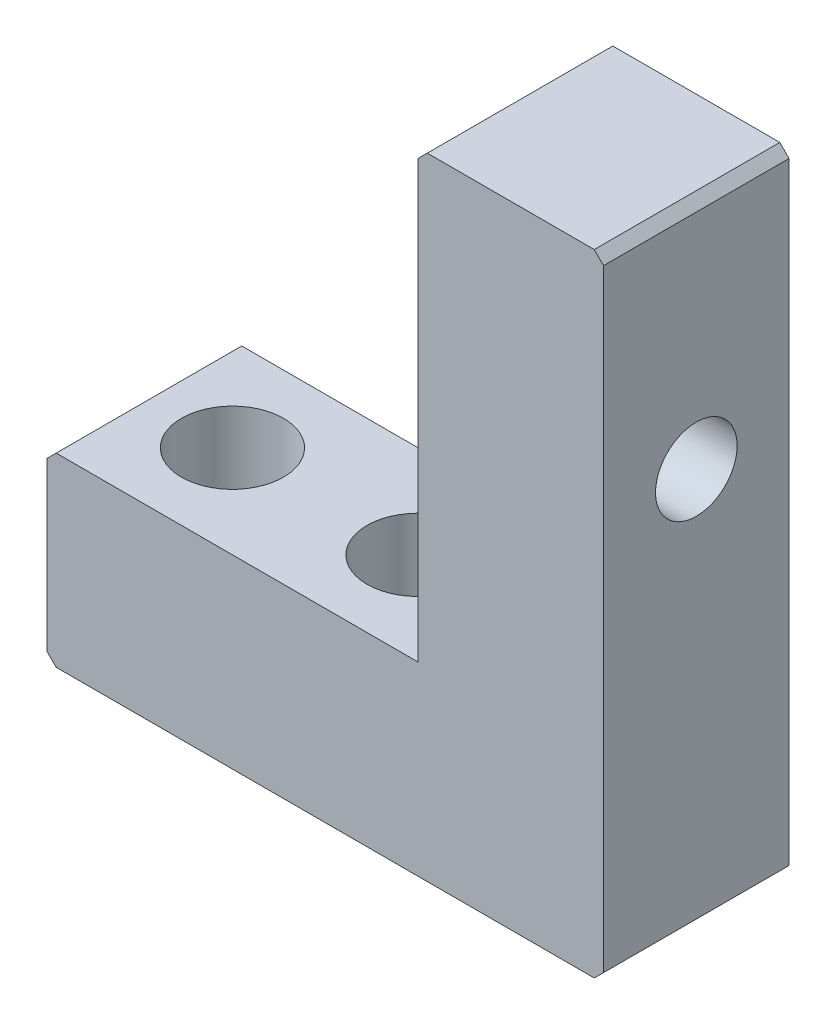
SolidWorks part; units mm, degrees
ref_plane "Front Plane" through (0, 0, 0) normal (0, 0, 1) x (1, 0, 0)
ref_plane "Top Plane" through (0, 0, 0) normal (0, 1, 0) x (1, 0, 0)
ref_plane "Right Plane" through (0, 0, 0) normal (1, 0, 0) x (0, 0, -1)
sketch "Sketch1" plane through (0, 0, 0) normal (0, 0, 1) x (1, 0, 0)
  line L0 (6.4361, 42.8739) -> (6.4361, -5.1261)
  line L1 (6.4361, -5.1261) -> (-33.5639, -5.1261)
  line L2 (-33.5639, -5.1261) -> (-33.5639, -25.1261)
  line L3 (-33.5639, -25.1261) -> (26.4361, -25.1261)
  line L4 (26.4361, -25.1261) -> (26.4361, 42.8739)
  line L5 (26.4361, 42.8739) -> (6.4361, 42.8739)
  dimension "D1" = 20
  dimension "D2" = 68
  dimension "D3" = 20
  dimension "D4" = 60
extrude "Boss-Extrude1" add sketch "Sketch1" along normal blind 20
sketch "Sketch2" plane through (6.4361, 0, 0) normal (-1, 0, 0) x (0, 0, 1)
  line L0 (20, -25.1261) -> (0, -25.1261) construction
  circle A0 centre (10, 17.8739) radius 3.5604
  dimension "D1" = 43
hole_wizard "M10x1.25 Tapped Hole1" positions "Sketch3" profile "Sketch4" tap size "M10x1.25" standard "GB" end condition through all
sketch "Sketch3" plane through (6.4361, 0, 0) normal (-1, 0, 0) x (0, 0, 1)
  point P0 (10, 17.8739)
sketch "Sketch4" plane through (6.4361, 17.8739, 10) normal (0, 1, 0) x (0, 0, 1)
  line L0 (0, 0) -> (0, 20)
  line L1 (0, 20) -> (4.4, 20)
  line L2 (4.4, 20) -> (4.4, 0)
  line L5 (4.4, 0) -> (0, 0)
  line L11 (0, -6.35) -> (0, 107.95) construction
  dimension "通孔螺纹孔钻头直径" = 8.8
  dimension "通孔螺纹孔钻头深度" = 20
cosmetic thread "Cosmetic thread 1" parameters "D2"=10
sketch "Sketch5" plane through (0, -5.1261, 0) normal (0, 1, 0) x (1, 0, 0)
  line L0 (-23.5639, -10) -> (-3.5639, -10)
  line L1 (-33.5639, -20) -> (-33.5639, 0) construction
  dimension "D1" = 20
  dimension "D2" = 10
hole_wizard "Hole1" positions "Sketch6" profile "Sketch7" legacy end condition through all
sketch "Sketch6" plane through (0, -5.1261, 0) normal (0, 1, 0) x (1, 0, 0)
  point P0 (-3.5639, -10)
  point P3 (-23.5639, -10)
sketch "Sketch7" plane through (-3.5639, -5.1261, 10) normal (1, 0, 0) x (0, 0, 1)
  line L0 (0, 0) -> (0, 20)
  line L1 (0, 20) -> (3.3, 20)
  line L2 (3.3, 20) -> (3.3, 10)
  line L3 (3.3, 10) -> (5.5, 10)
  line L4 (5.5, 10) -> (5.5, 0)
  line L5 (5.5, 0) -> (0, 0)
  line L6 (0, 110) -> (0, -10) construction
  dimension "直径" = 6.6
  dimension "深度" = 20
  dimension "柱坑直径" = 11
  dimension "柱坑深度" = 10
chamfer "Chamfer1" distance 1 angle 45 5 edges at (26.4361, -25.1261, 10) (-33.5639, -25.1261, 10) (-33.5639, -5.1261, 10) (6.4361, 42.8739, 10) (26.4361, 42.8739, 10)
